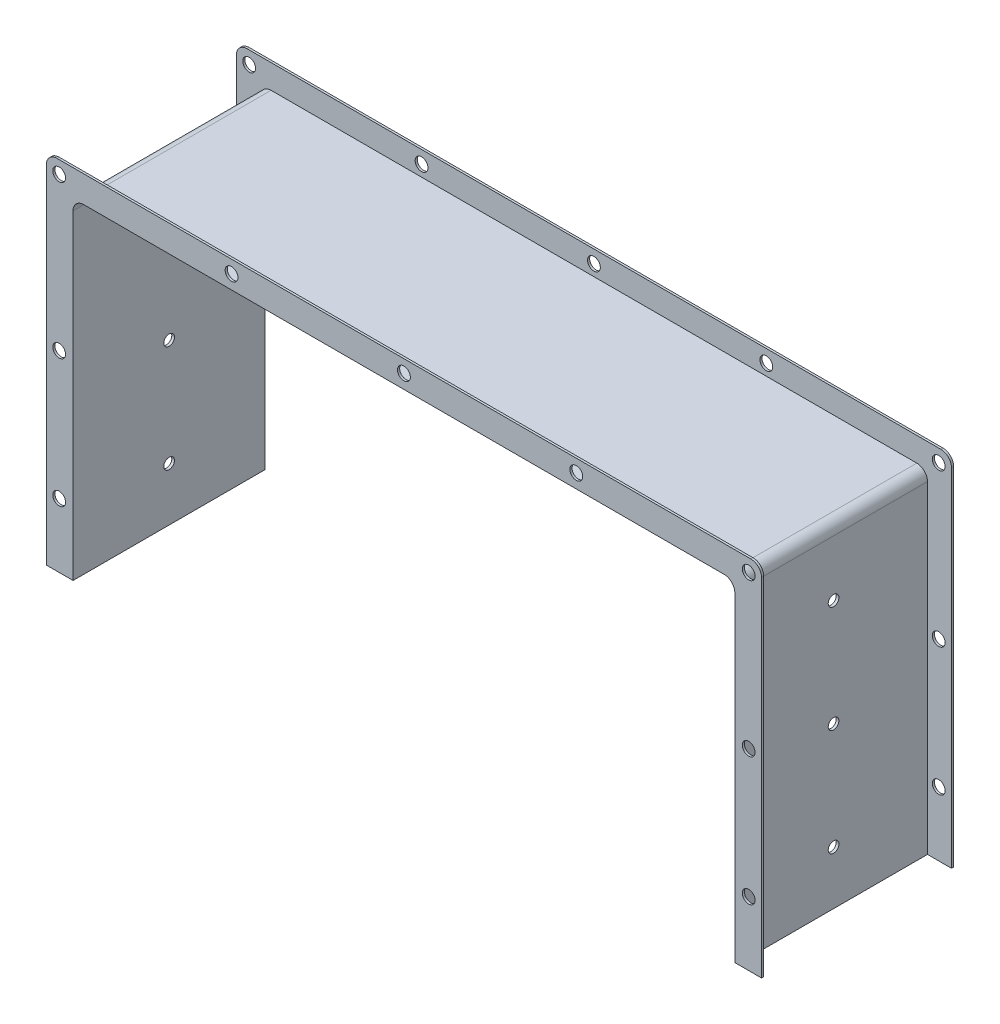
from build123d import *

# Parameters (mm, degrees)
BOSS_EXTRUDE1_DEPTH     = 2
BOSS_EXTRUDE2_START     = 178
BOSS_EXTRUDE2_DEPTH     = 178
CUT_EXTRUDE1_DEPTH      = 415.686930105
CUT_EXTRUDE1_DEPTH_BACK = 415.686930105
SKETCH3_R               = 6
SKETCH4_R               = 5
CUT_EXTRUDE2_DEPTH      = 693.095730373
SKETCH5_R               = 6
BOSS_EXTRUDE3_DEPTH     = 2


with BuildPart() as part:
    # Sketch1 → Boss-Extrude1 (new body)
    with BuildSketch(Plane.XY):
        with BuildLine():
            Line((-335, -167.5), (-335, 157.5))
            ThreePointArc((-335, 157.5), (-332.071067812, 164.571067812), (-325, 167.5))
            Line((-325, 167.5), (325, 167.5))
            ThreePointArc((325, 167.5), (332.071067812, 164.571067812), (335, 157.5))
            Line((335, 157.5), (335, -167.5))
            Line((335, -167.5), (310, -167.5))
            Line((310, -167.5), (310, 132.5))
            ThreePointArc((310, 132.5), (307.071067812, 139.571067812), (300, 142.5))
            Line((300, 142.5), (-300, 142.5))
            ThreePointArc((-300, 142.5), (-307.071067812, 139.571067812), (-310, 132.5))
            Line((-310, 132.5), (-310, -167.5))
            Line((-310, -167.5), (-335, -167.5))
        make_face()
    extrude(amount=BOSS_EXTRUDE1_DEPTH)

    # Sketch2 → Boss-Extrude2 (add)
    with BuildSketch(Plane(origin=(0, 0, 0), x_dir=(-1, 0, 0), z_dir=(0, 0, -1)).offset(BOSS_EXTRUDE2_START)):
        with BuildLine():
            Line((310, -167.5), (310, 132.5))
            ThreePointArc((310, 132.5), (307.071067812, 139.571067812), (300, 142.5))
            Line((300, 142.5), (-300, 142.5))
            ThreePointArc((-300, 142.5), (-307.071067812, 139.571067812), (-310, 132.5))
            Line((-310, 132.5), (-310, -167.5))
            Line((-310, -167.5), (-312.5, -167.5))
            Line((-312.5, -167.5), (-312.5, 135))
            ThreePointArc((-312.5, 135), (-309.571067812, 142.071067812), (-302.5, 145))
            Line((-302.5, 145), (302.5, 145))
            ThreePointArc((302.5, 145), (309.571067812, 142.071067812), (312.5, 135))
            Line((312.5, 135), (312.5, -167.5))
            Line((312.5, -167.5), (310, -167.5))
        make_face()
    extrude(amount=-BOSS_EXTRUDE2_DEPTH)

    # Sketch3 → Cut-Extrude1 (cut, two sides: drawn at the far end of the back side and taken through both)
    with BuildSketch(Plane(origin=(0, 0, 0), x_dir=(-1, 0, 0), z_dir=(0, 0, -1)).offset(-CUT_EXTRUDE1_DEPTH_BACK)):
        with Locations((0, 155.5)):
            Circle(SKETCH3_R)
        with Locations((-161.5, 155.5)):
            Circle(SKETCH3_R)
        with Locations((-323, 12.5)):
            Circle(SKETCH3_R)
        with Locations((-323, -107.5)):
            Circle(SKETCH3_R)
        with Locations((-323, 155.5)):
            Circle(SKETCH3_R)
        with Locations((323, 155.5)):
            Circle(SKETCH3_R)
        with Locations((323, -107.5)):
            Circle(SKETCH3_R)
        with Locations((323, 12.5)):
            Circle(SKETCH3_R)
        with Locations((161.5, 155.5)):
            Circle(SKETCH3_R)
    extrude(amount=CUT_EXTRUDE1_DEPTH + CUT_EXTRUDE1_DEPTH_BACK, mode=Mode.SUBTRACT)

    # Sketch4 → Cut-Extrude2 (cut, through all)
    with BuildSketch(Plane(origin=(312.5, 0, 0), x_dir=(0, 0, -1), z_dir=(1, 0, 0))):
        with Locations((88, 82.5)):
            Circle(SKETCH4_R)
        with Locations((88, -17.5)):
            Circle(SKETCH4_R)
        with Locations((88, -117.5)):
            Circle(SKETCH4_R)
    extrude(amount=-CUT_EXTRUDE2_DEPTH, mode=Mode.SUBTRACT)

    # Sketch5 → Boss-Extrude3 (add)
    with BuildSketch(Plane(origin=(0, 0, -178), x_dir=(-1, 0, 0), z_dir=(0, 0, -1))):
        with BuildLine():
            Line((-312.5, -167.5), (-312.5, 135))
            ThreePointArc((-312.5, 135), (-309.571067812, 142.071067812), (-302.5, 145))
            Line((-302.5, 145), (302.5, 145))
            ThreePointArc((302.5, 145), (309.571067812, 142.071067812), (312.5, 135))
            Line((312.5, 135), (312.5, -167.5))
            Line((312.5, -167.5), (335, -167.5))
            Line((335, -167.5), (335, 157.5))
            ThreePointArc((335, 157.5), (332.071067812, 164.571067812), (325, 167.5))
            Line((325, 167.5), (-325, 167.5))
            ThreePointArc((-325, 167.5), (-332.071067812, 164.571067812), (-335, 157.5))
            Line((-335, 157.5), (-335, -167.5))
            Line((-335, -167.5), (-312.5, -167.5))
        make_face()
        with Locations((-323, -107.5)):
            Circle(SKETCH5_R, mode=Mode.SUBTRACT)
        with Locations((-323, 12.5)):
            Circle(SKETCH5_R, mode=Mode.SUBTRACT)
        with Locations((-161.5, 155.5)):
            Circle(SKETCH5_R, mode=Mode.SUBTRACT)
        with Locations((0, 155.5)):
            Circle(SKETCH5_R, mode=Mode.SUBTRACT)
        with Locations((161.5, 155.5)):
            Circle(SKETCH5_R, mode=Mode.SUBTRACT)
        with Locations((323, 12.5)):
            Circle(SKETCH5_R, mode=Mode.SUBTRACT)
        with Locations((323, -107.5)):
            Circle(SKETCH5_R, mode=Mode.SUBTRACT)
        with Locations((323, 155.5)):
            Circle(SKETCH5_R, mode=Mode.SUBTRACT)
        with Locations((-323, 155.5)):
            Circle(SKETCH5_R, mode=Mode.SUBTRACT)
    extrude(amount=-BOSS_EXTRUDE3_DEPTH)


solid = part.part
